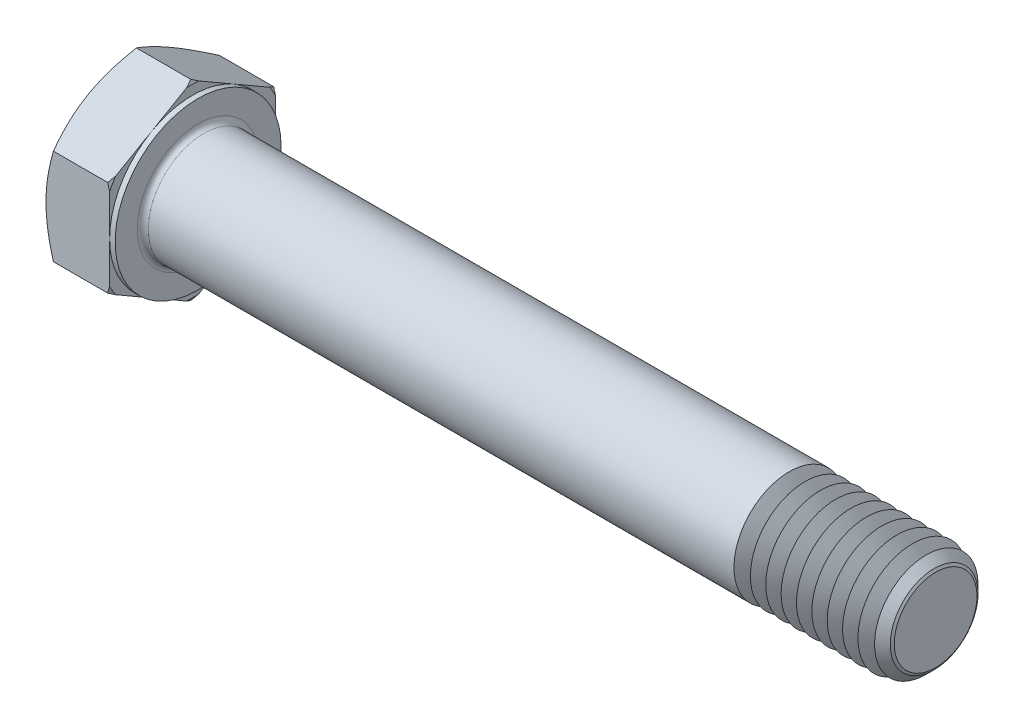
from build123d import *

# Parameters (mm, degrees)
EXTRUDE_364_DEPTH      = 7.5
SKETCH_4_W             = 0.6
SKETCH_4_H             = 11.392304845
CHAMFER_2049_SIZE      = 1.4
FILLET_2094_R          = 0.6
PATTERN_LINEAR_1_COUNT = 10
PATTERN_LINEAR_1_PITCH = 1.666666667


with BuildPart() as part:
    # 草图1 → Extrude 364 (new body)
    with BuildSketch(Plane(origin=(0, 0, 0), x_dir=(0, 0, -1), z_dir=(1, 0, 0))):
        Polygon((9, 5.196152423), (9, -5.196152423), (0, -10.392304845), (-9, -5.196152423), (-9, 5.196152423), (0, 10.392304845), align=None)
    extrude(amount=EXTRUDE_364_DEPTH)

    # 草图2 → 凸台-旋转1 (revolve)
    with BuildSketch(Plane.XY, mode=Mode.PRIVATE) as revolve_1_sk:
        Polygon((0, 0), (87.5, 0), (87.5, 4.4845), (87.5, 6), (7.791693541, 6), (0, 6), align=None)
    revolve(revolve_1_sk.sketch.rotate(Axis((0, 0, 0), (1, 0, 0)), 90), axis=Axis((0, 0, 0), (1, 0, 0)))

    # 草图3 → 切除-旋转1 (revolve, cut)
    with BuildSketch(Plane.XY):
        Polygon((0, 9), (3.690598923, 15.392304845), (3.690598923, 20.392304845), (-10, 20.392304845), (-10, 9), align=None)
    revolve(axis=Axis((0, 0, 0), (1, 0, 0)), mode=Mode.SUBTRACT)

    # 草图5 → 切除-旋转2 (revolve, cut)
    with BuildSketch(Plane.XY):
        Polygon((7.5, 9), (3.809401077, 15.392304845), (3.809401077, 20.392304845), (13.809401077, 20.392304845), (13.809401077, 9), align=None)
    revolve(axis=Axis((0, 0, 0), (1, 0, 0)), mode=Mode.SUBTRACT)

    # 草图4 → 切除-旋转3 (revolve, cut)
    with BuildSketch(Plane.XY, mode=Mode.PRIVATE) as cut_revolve_3_sk:
        with Locations((7.2, 14.696152423)):
            Rectangle(SKETCH_4_W, SKETCH_4_H)
    revolve(cut_revolve_3_sk.sketch.rotate(Axis((0, 0, 0), (1, 0, 0)), 270), axis=Axis((0, 0, 0), (1, 0, 0)), mode=Mode.SUBTRACT)

    # Chamfer 2049
    chamfer_2049_edges = [part.edges().sort_by_distance(p)[0] for p in [
        (87.5, 0, -6),
    ]]
    chamfer(chamfer_2049_edges, length=CHAMFER_2049_SIZE)

    # Fillet 2094
    fillet_2094_edges = [part.edges().sort_by_distance(p)[0] for p in [
        (7.5, 0, -6),
    ]]
    fillet(fillet_2094_edges, radius=FILLET_2094_R)

    # 草图6 → 切除-旋转4 (revolve, cut)
    with BuildSketch(Plane.XY):
        Polygon((72.5, -4.4845), (71.625025667, -6), (71.625025667, -7.5), (73.374974333, -7.5), (73.374974333, -6), align=None)
    cut_revolve_4 = revolve(axis=Axis((-3.175, 0, 0), (1, 0, 0)), mode=Mode.SUBTRACT)

    # 阵列(线性)1: 切除-旋转4 ×10
    with Locations(*[(i * PATTERN_LINEAR_1_PITCH, 0, 0) for i in range(1, PATTERN_LINEAR_1_COUNT)]):
        add(cut_revolve_4, mode=Mode.SUBTRACT)


solid = part.part
